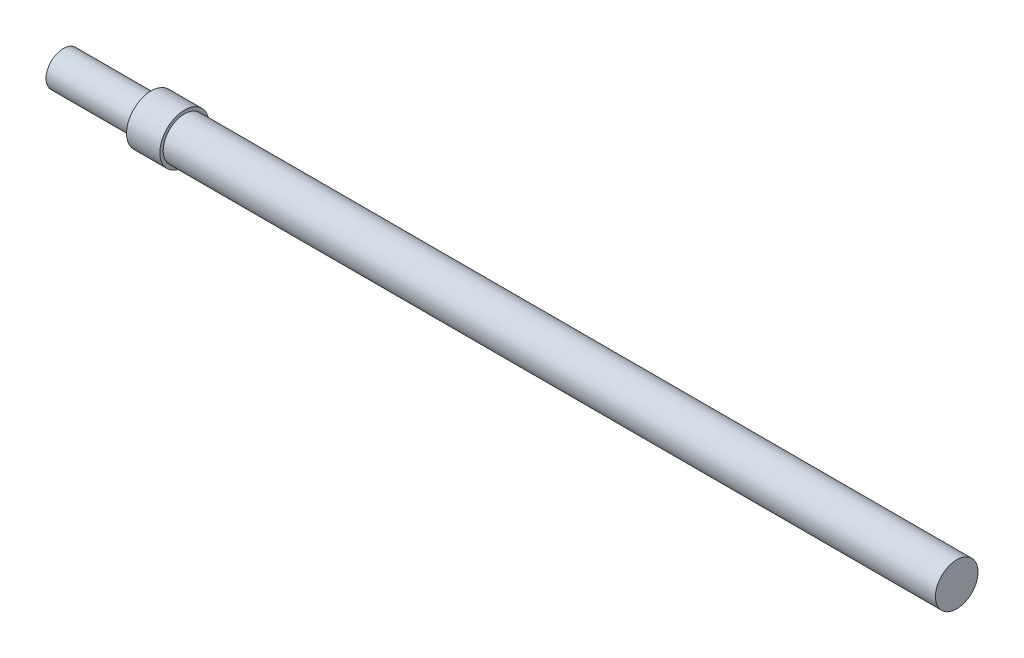
SolidWorks part; units mm, degrees
ref_plane "前视基准面" through (0, 0, 0) normal (0, 0, 1) x (1, 0, 0)
ref_plane "上视基准面" through (0, 0, 0) normal (0, 1, 0) x (1, 0, 0)
ref_plane "右视基准面" through (0, 0, 0) normal (1, 0, 0) x (0, 0, -1)
other "Configuration Table"
sketch "草图1" plane through (0, 0, 0) normal (0, 0, 1) x (1, 0, 0)
  line L0 (-87.3026, 0) -> (425.6683, 0) construction
  line L1 (-81.3975, 0) -> (-81.3975, 13)
  line L2 (-81.3975, 13) -> (-15.3975, 13)
  line L3 (-15.3975, 13) -> (-15.3975, 18.5)
  line L4 (-15.3975, 18.5) -> (9.6025, 18.5)
  line L5 (9.6025, 18.5) -> (9.6025, 16)
  line L6 (589.6025, 16) -> (9.6025, 16)
  line L7 (589.6025, 16) -> (589.6025, 0)
  line L8 (-81.3975, 0) -> (589.6025, 0)
  dimension "D1" = 580
revolve "旋转1" add sketch "草图1" angle 360 about L0
